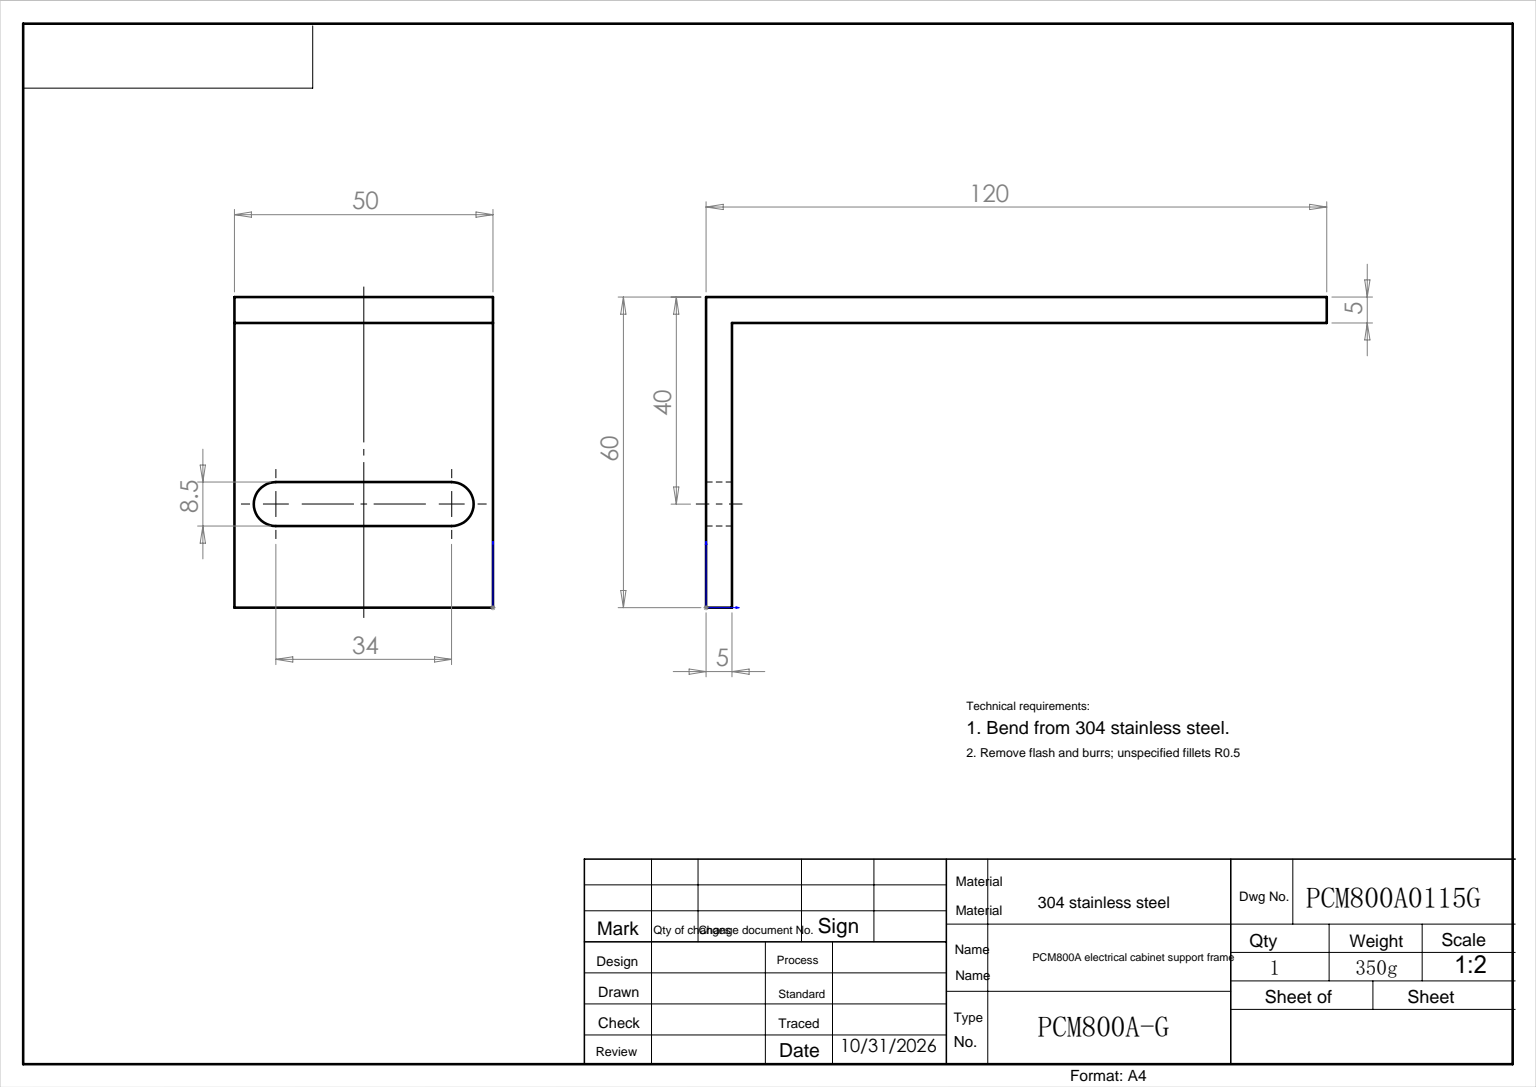
from build123d import *

# Parameters (mm, degrees)
EXTRUDE_1_DEPTH     = 50
CUT_EXTRUDE_1_DEPTH = 10


with BuildPart() as part:
    # 草图1 → 拉伸-薄壁1 (new body)
    with BuildSketch(Plane.XY):
        Polygon((0, 0), (0, 60), (120, 60), (120, 55), (5, 55), (5, 0), align=None)
    extrude(amount=EXTRUDE_1_DEPTH)

    # 草图2 → 切除-拉伸1 (cut)
    with BuildSketch(Plane.ZY):
        with BuildLine():
            Line((8, 24.25), (42, 24.25))
            ThreePointArc((42, 24.25), (46.25, 20), (42, 15.75))
            Line((42, 15.75), (8, 15.75))
            ThreePointArc((8, 15.75), (3.75, 20), (8, 24.25))
        make_face()
    extrude(amount=-CUT_EXTRUDE_1_DEPTH, mode=Mode.SUBTRACT)


solid = part.part
